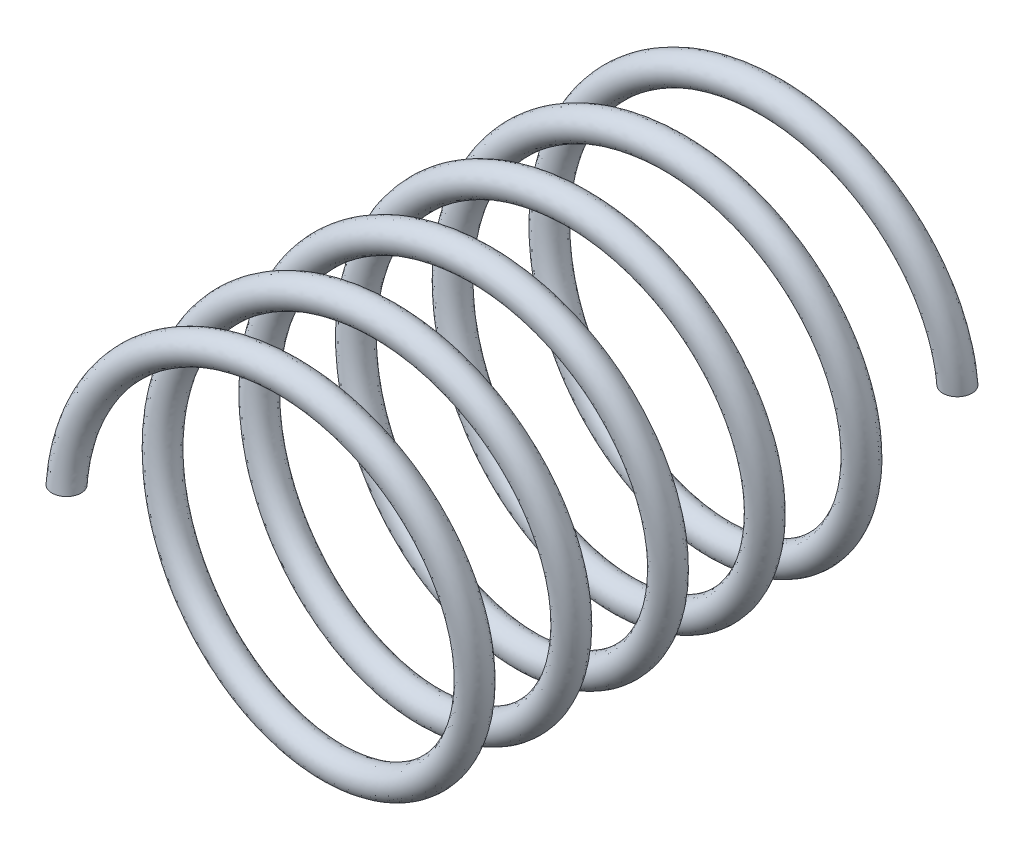
from build123d import *

# Parameters (mm, degrees)
SWEEP1_PITCH  = 14.95
SWEEP1_HEIGHT = 82.225
SWEEP1_RADIUS = 30
SKETCH2_R     = 2.25


with BuildPart() as part:
    # Sweep1: sweep along a helix
    with BuildLine() as sweep1_path:
        Helix(SWEEP1_PITCH, SWEEP1_HEIGHT, SWEEP1_RADIUS, center=(0, 0, 0), direction=(0, 0, 1))
    # Sketch2 → Sweep1 (sweep)
    with BuildSketch(Plane(origin=(0, 0, 0), x_dir=(1, 0, 0), z_dir=(0, 1, 0))):
        with Locations((27.75, 0)):
            Circle(SKETCH2_R)
    sweep(path=sweep1_path.line, is_frenet=True)


solid = part.part
